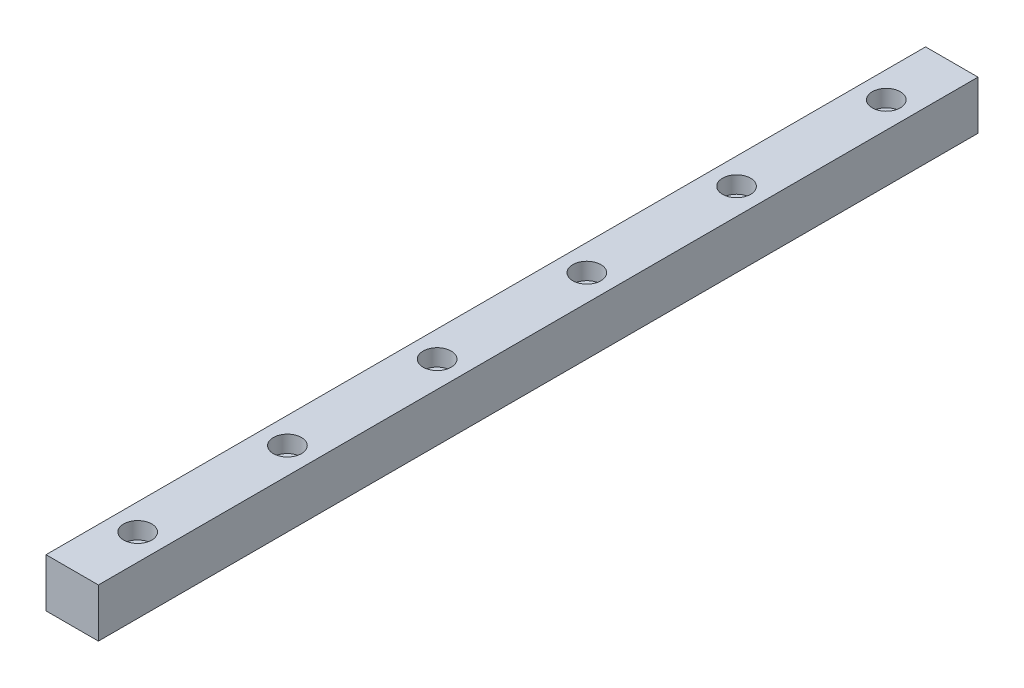
from build123d import *

# Parameters (mm, degrees)
SKETCH1_W                                            = 28
SKETCH1_H                                            = 26
BOSS_EXTRUDE1_DEPTH                                  = 470
HOLE_SIZE_PER_SOCKET_HEAD_CAP_SCREW_TYPE_D           = 9
HOLE_SIZE_PER_SOCKET_HEAD_CAP_SCREW_TYPE_CBORE_D     = 15
HOLE_SIZE_PER_SOCKET_HEAD_CAP_SCREW_TYPE_CBORE_DEPTH = 9
LPATTERN1_COUNT                                      = 6
LPATTERN1_PITCH                                      = 80


with BuildPart() as part:
    # Sketch1 → Boss-Extrude1 (new body)
    with BuildSketch(Plane.XY):
        Rectangle(SKETCH1_W, SKETCH1_H)
    extrude(amount=-BOSS_EXTRUDE1_DEPTH)

    # Hole size per socket head cap screw type1 (through all)
    with Locations(Plane(origin=(0, 13, 0), x_dir=(-1, 0, 0), z_dir=(0, 1, 0))):
        with Locations((0, -35)):
            hole_size_per_socket_head_cap_screw_type = CounterBoreHole(HOLE_SIZE_PER_SOCKET_HEAD_CAP_SCREW_TYPE_D / 2, HOLE_SIZE_PER_SOCKET_HEAD_CAP_SCREW_TYPE_CBORE_D / 2, HOLE_SIZE_PER_SOCKET_HEAD_CAP_SCREW_TYPE_CBORE_DEPTH)

    # LPattern1: Hole size per socket head cap screw type1 ×6
    with Locations(*[(0, 0, -i * LPATTERN1_PITCH) for i in range(1, LPATTERN1_COUNT)]):
        add(hole_size_per_socket_head_cap_screw_type, mode=Mode.SUBTRACT)


solid = part.part
